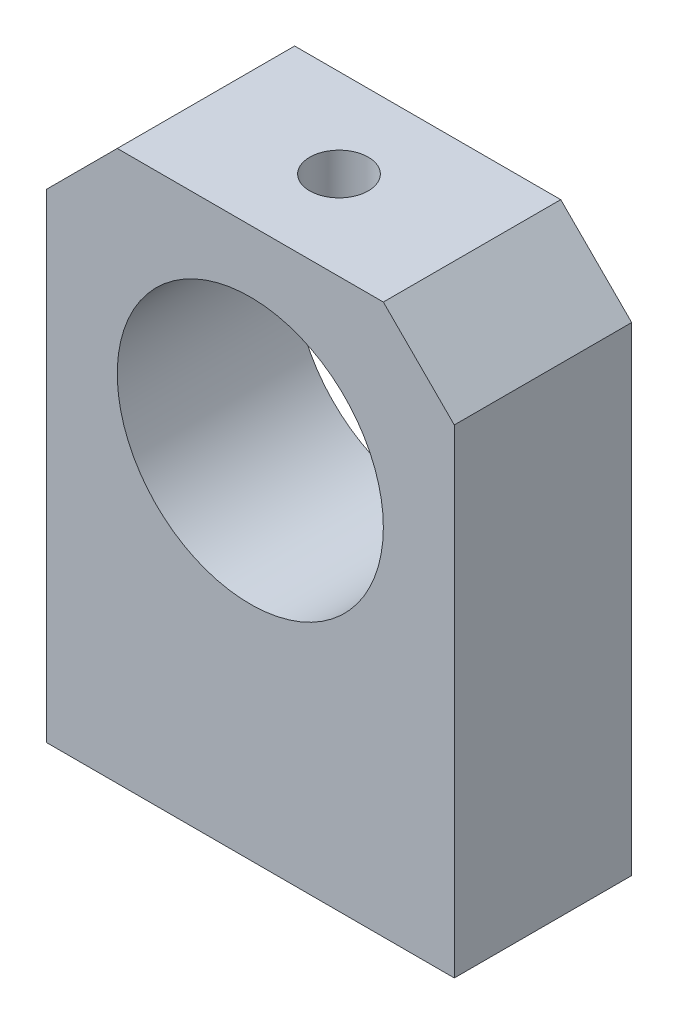
SolidWorks part; units mm, degrees
ref_plane "前视基准面" through (0, 0, 0) normal (0, 0, 1) x (1, 0, 0)
ref_plane "上视基准面" through (0, 0, 0) normal (0, 1, 0) x (1, 0, 0)
ref_plane "右视基准面" through (0, 0, 0) normal (1, 0, 0) x (0, 0, -1)
sketch "草图1" plane through (0, 0, 0) normal (0, 0, 1) x (1, 0, 0)
  line L3 (-11.5, 0) -> (-11.5, 31)
  line L4 (-11.5, 31) -> (11.5, 31)
  line L5 (11.5, 31) -> (11.5, 0)
  line L9 (-11.5, 0) -> (11.5, 0)
  circle A0 centre (0, 20) radius 7.5
  dimension "D3" = 15
  dimension "D1" = 20
  dimension "D4" = 23
  dimension "D5" = 11
extrude "凸台-拉伸1" add sketch "草图1" along normal mid plane 10
sketch "草图2" plane through (0, 0, 5) normal (0, 0, 1) x (1, 0, 0)
  line L0 (11.5, 31) -> (-11.5, 31) construction
  line L1 (-1, 31) -> (1, 31)
  line L2 (-1, 31) -> (-1, 27.433)
  line L3 (-1, 27.433) -> (1, 27.433)
  line L4 (1, 31) -> (1, 27.433)
  circle A0 centre (0, 20) radius 7.5 construction
  dimension "D1" = 2
extrude "切除-拉伸1" [suppressed] cut sketch "草图2" against normal up to next
sketch "草图4" plane through (11.5, 0, 0) normal (1, 0, 0) x (0, 0, -1)
  line L0 (-5, 31) -> (5, 31) construction
  circle A0 centre (0, 26) radius 3
  dimension "D1" = 6
  dimension "D2" = 5
extrude "切除-拉伸2" [suppressed] cut sketch "草图4" against normal up to next
hole_wizard "M5 螺纹孔1" positions "3D草图1" profile "草图5" tap size "M5" standard "GB"
sketch3d "3D草图1" [suppressed]
  circle A0 centre (11.5, 31, 0) radius 3 construction
  point P0 (-1, 31, 0)
  point P4 (14.5, 31, 0)
sketch "草图5" plane through (-1, 31, 0) normal (0, 1, 0) x (0, 0, -1)
  line L0 (0, 0) -> (0, 10.5)
  line L1 (0, 10.5) -> (2.1, 10.5)
  line L2 (2.1, 10.5) -> (2.1, 0)
  line L5 (2.1, 0) -> (0, 0)
  line L11 (0, -6.35) -> (0, 107.95) construction
  dimension "通孔螺纹孔钻头直径" = 4.2
  dimension "通孔螺纹孔钻头深度" = 10.5
cosmetic thread "孔螺蚊线1" [suppressed] parameters "D2"=5
chamfer "倒角1" distance 4 angle 45 2 edges at (-11.5, 31, 0) (11.5, 31, 0)
hole_wizard "M4 螺纹孔1" positions "3D草图2" profile "草图7" tap size "M4" standard "GB"
sketch3d "3D草图2"
  line L0 (0, 31, -5) -> (0, 31, 5)
  line L1 (7.5, 31, -5) -> (-7.5, 31, -5) construction
  line L2 (7.5, 31, 5) -> (-7.5, 31, 5) construction
  point P0 (0, 31, 0)
sketch "草图7" plane through (0, 31, 0) normal (1, 0, 0) x (0, 0, 1)
  line L0 (0, 0) -> (0, 3.5)
  line L1 (0, 3.5) -> (1.65, 3.5)
  line L2 (1.65, 3.5) -> (1.65, 0)
  line L5 (1.65, 0) -> (0, 0)
  line L11 (0, -6.35) -> (0, 107.95) construction
  dimension "通孔螺纹孔钻头直径" = 3.3
  dimension "通孔螺纹孔钻头深度" = 3.5
cosmetic thread "孔螺蚊线2" parameters "D2"=4
hole_wizard "M5 螺纹孔2" positions "3D草图3" profile "草图8" tap size "M5" standard "GB"
sketch3d "3D草图3"
  line L0 (11.5, 0, 0) -> (-11.5, 0, 0)
  line L1 (11.5, 0, 5) -> (11.5, 0, -5) construction
  line L2 (-11.5, 0, 5) -> (-11.5, 0, -5) construction
  point P0 (-6.5, 0, 0)
  point P2 (6.5, 0, 0)
  dimension "D1" = 5
  dimension "D2" = 5
sketch "草图8" plane through (-6.5, 0, 0) normal (1, 0, 0) x (0, 0, -1)
  line L0 (0, 0) -> (0, 9.6618)
  line L1 (0, 9.6618) -> (2.1, 8.4)
  line L2 (2.1, 8.4) -> (2.1, 0)
  line L5 (2.1, 0) -> (0, 0)
  line L10 (0, 9.6618) -> (-2.1, 8.4) construction
  line L11 (0, -6.35) -> (0, 107.95) construction
  dimension "螺纹孔钻头直径" = 4.2
  dimension "螺纹孔钻头深度" = 8.4
  dimension "导头角度" = 118
cosmetic thread "孔螺蚊线3" parameters "D1"=6, "D2"=5
cosmetic thread "孔螺蚊线4" parameters "D1"=6, "D2"=5
